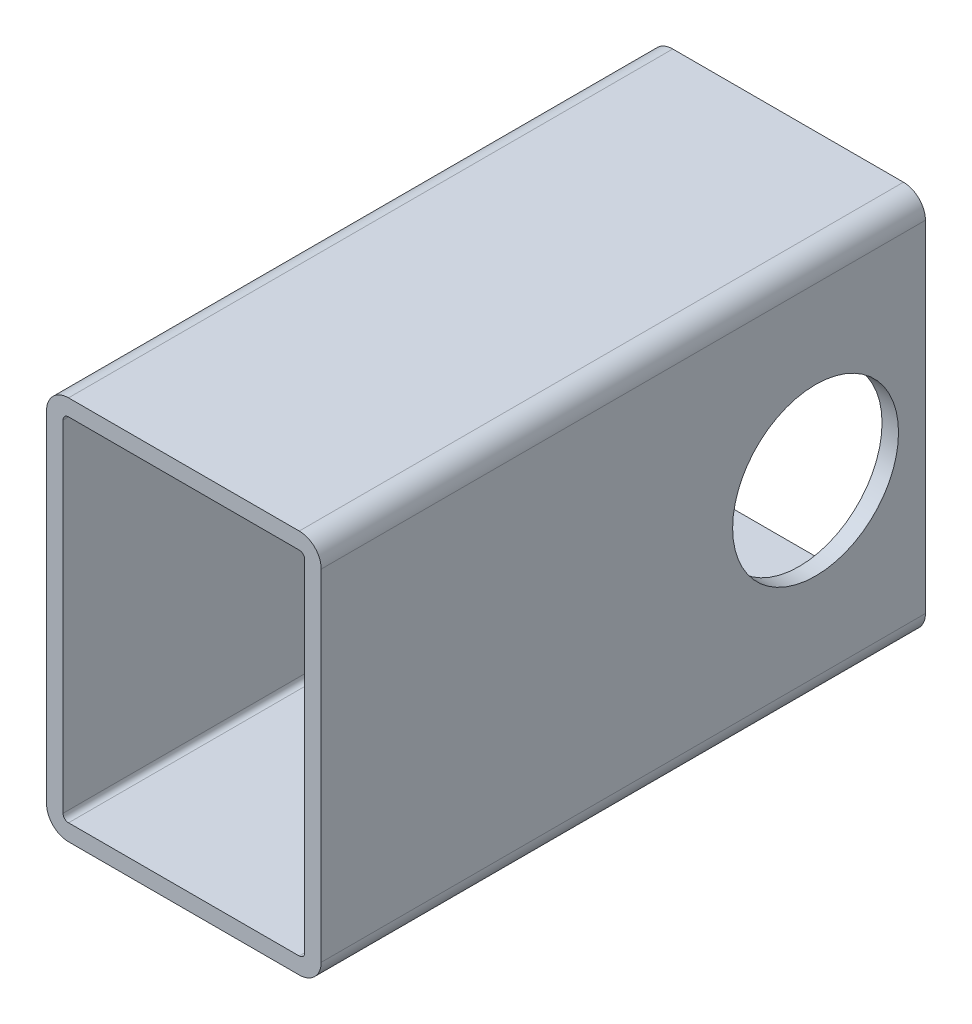
SolidWorks part; units mm, degrees
material "AISI 1045 钢，冷拔"
ref_plane "Front Plane" through (0, 0, 0) normal (0, 0, 1) x (1, 0, 0)
ref_plane "Top Plane" through (0, 0, 0) normal (0, 1, 0) x (1, 0, 0)
ref_plane "Right Plane" through (0, 0, 0) normal (1, 0, 0) x (0, 0, -1)
sketch "Sketch1" plane through (0, 0, 0) normal (0, 0, 1) x (1, 0, 0)
  line L1 (-21, -35) -> (21, -35)
  line L2 (-25, -31) -> (-25, 31)
  line L3 (-21, 35) -> (21, 35)
  line L4 (25, -31) -> (25, 31)
  line L5 (-25, -35) -> (25, 35) construction
  line L6 (-25, 35) -> (25, -35) construction
  arc A0 (-21, -35) -> (-25, -31) centre (-21, -31) cw
  arc A1 (21, -35) -> (25, -31) centre (21, -31) ccw
  arc A2 (21, 35) -> (25, 31) centre (21, 31) cw
  arc A3 (-25, 31) -> (-21, 35) centre (-21, 31) cw
  point P0 (0, 0)
  dimension "D3" = 4
  dimension "D1" = 50
  dimension "D2" = 70
extrude "Extrude-Thin1" add sketch "Sketch1" along normal blind 110 thin thin type one direction reverse wall 3
sketch "Sketch2" plane through (25, 0, 0) normal (1, 0, 0) x (0, 0, -1)
  line L0 (0, -31) -> (0, 31) construction
  line L1 (-110, 35) -> (0, 35) construction
  circle A0 centre (-20, 0) radius 15.1
  dimension "D1" = 30.2
  dimension "D2" = 20
  dimension "D3" = 35
extrude "Cut-Extrude1" cut sketch "Sketch2" against normal through all
